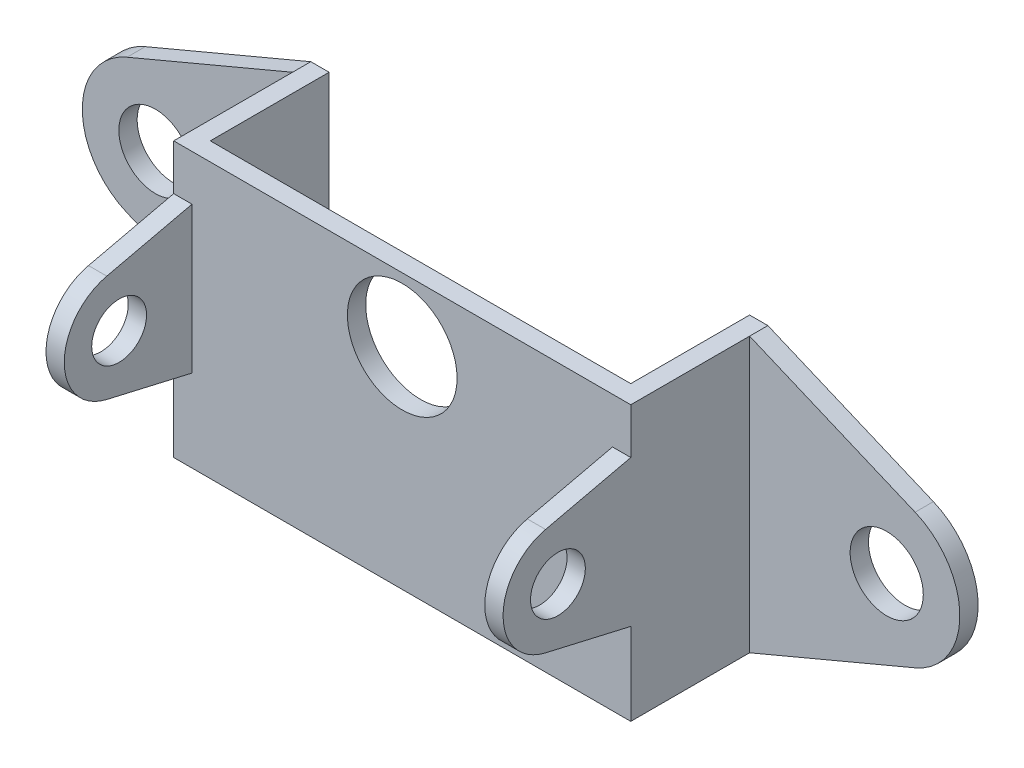
from build123d import *

# Parameters (mm, degrees)
SKETCH1_R             = 2
BOSS_EXTRUDE1_DEPTH   = 1
BOSS_EXTRUDE1_2_DEPTH = 1
SKETCH2_W             = 1
SKETCH2_H             = 15
BOSS_EXTRUDE2_DEPTH   = 6.5
SKETCH4_W             = 24.99999999
SKETCH4_H             = 15
SKETCH4_R             = 3
BOSS_EXTRUDE3_DEPTH   = 1
SKETCH6_R             = 1.5
BOSS_EXTRUDE4_DEPTH   = 1
CUT_EXTRUDE1_DEPTH    = 1
SKETCH8_R             = 1.5
BOSS_EXTRUDE5_DEPTH   = 1


with BuildPart() as part:
    # Sketch1 → Boss-Extrude1 (new body)
    with BuildSketch(Plane.XY):
        with BuildLine():
            Line((-99.978251459, 146.432775889), (-109.031169153, 142.619026916))
            Line((-109.031169153, 142.619026916), (-109.031169153, 157.619026916))
            Line((-109.031169153, 157.619026916), (-99.978251459, 153.805277943))
            ThreePointArc((-99.978251459, 153.805277943), (-97.531169153, 150.119026916), (-99.978251459, 146.432775889))
        make_face()
        with Locations((-101.531169153, 150.119026916)):
            Circle(SKETCH1_R, mode=Mode.SUBTRACT)
    extrude(amount=BOSS_EXTRUDE1_DEPTH)

    # Sketch2 → Boss-Extrude2 (add)
    with BuildSketch(Plane.XY):
        with Locations((-109.531169153, 150.119026916)):
            Rectangle(SKETCH2_W, SKETCH2_H)
        with Locations((-133.531169143, 150.119026916)):
            Rectangle(SKETCH2_W, SKETCH2_H)
    extrude(amount=BOSS_EXTRUDE2_DEPTH)


with BuildPart() as body_2:
    # Sketch1 → Boss-Extrude1 2 (new body)
    with BuildSketch(Plane.XY):
        with BuildLine():
            Line((-143.084086847, 153.805277943), (-134.031169153, 157.619026916))
            Line((-134.031169153, 157.619026916), (-134.031169153, 142.619026916))
            Line((-134.031169153, 142.619026916), (-143.084086847, 146.432775889))
            ThreePointArc((-143.084086847, 146.432775889), (-145.531169153, 150.119026916), (-143.084086847, 153.805277943))
        make_face()
        with Locations(Location((-141.531169153, 150.119026916, 0), (0, 0, 180))):
            Circle(SKETCH1_R, mode=Mode.SUBTRACT)
    extrude(amount=BOSS_EXTRUDE1_2_DEPTH)


with BuildPart() as boss_extrude2_piece_1:
    # of the separate pieces the step leaves, piece 1, a body of its own (boss_extrude2_pieces)
    add(part.part.solids().sort_by_distance((-99.978251459, 146.432775889, 0))[0])

    # Sketch4 → Boss-Extrude3 (add)
    with BuildSketch(Plane.XY.offset(6.5)):
        with Locations((-121.531169148, 150.119026916)):
            Rectangle(SKETCH4_W, SKETCH4_H)
        with Locations((-121.531169153, 154.119026916)):
            Circle(SKETCH4_R, mode=Mode.SUBTRACT)
    extrude(amount=BOSS_EXTRUDE3_DEPTH)



with BuildPart() as boss_extrude2_piece_2:
    # of the separate pieces the step leaves, piece 2, a body of its own (boss_extrude2_pieces)
    add(part.part.solids().sort_by_distance((-134.031169143, 157.619026916, 0))[0])


with BuildPart() as boss_extrude2_piece_1_1:
    add(boss_extrude2_piece_1.part)

    add(boss_extrude2_piece_2.part)  # Boss-Extrude4 merges Boss-Extrude2 piece 2
    # Sketch6 → Boss-Extrude4 (add)
    with BuildSketch(Plane.ZY.offset(134.031169143)):
        with BuildLine():
            Line((11.484935003, 147.119026916), (5.675712497, 147.119026916))
            ThreePointArc((5.675712497, 147.119026916), (1.675712497, 151.119026916), (5.675712497, 155.119026916))
            Line((5.675712497, 155.119026916), (11.484935003, 155.119026916))
            ThreePointArc((11.484935003, 155.119026916), (15.484935003, 151.119026916), (11.484935003, 147.119026916))
        make_face()
        with Locations((11.484935003, 151.119026916)):
            Circle(SKETCH6_R, mode=Mode.SUBTRACT)
    extrude(amount=-BOSS_EXTRUDE4_DEPTH)

    # Sketch7 → Cut-Extrude1 (cut)
    with BuildSketch(Plane.ZY.offset(134.031169143)):
        with BuildLine():
            Line((12.160438985, 154.041986781), (7.5, 155.119026916))
            Line((7.5, 155.119026916), (10.709914087, 160.89800408))
            Line((10.709914087, 160.89800408), (15.340416768, 156.67870434))
            Line((15.340416768, 156.67870434), (15.715862932, 151.386701277))
            Line((15.715862932, 151.386701277), (14.535889275, 146.058941435))
            Line((14.535889275, 146.058941435), (7.5, 147.119026916))
            Line((7.5, 147.119026916), (12.160438985, 148.196067051))
            ThreePointArc((12.160438985, 148.196067051), (14.484935003, 151.119026916), (12.160438985, 154.041986781))
        make_face()
    extrude(amount=-CUT_EXTRUDE1_DEPTH, mode=Mode.SUBTRACT)

    # Sketch8 → Boss-Extrude5 (add)
    with BuildSketch(Plane(origin=(-109.031169153, 0, 0), x_dir=(0, 0, -1), z_dir=(1, 0, 0))):
        with BuildLine():
            Line((-7.5, 147.119026916), (-7.5, 155.119026916))
            Line((-7.5, 155.119026916), (-12.160438985, 154.041986781))
            ThreePointArc((-12.160438985, 154.041986781), (-14.484935003, 151.119026916), (-12.160438985, 148.196067051))
            Line((-12.160438985, 148.196067051), (-7.5, 147.119026916))
        make_face()
        with Locations(Location((-11.484935003, 151.119026916, 0), (0, 0, 180))):
            Circle(SKETCH8_R, mode=Mode.SUBTRACT)
    extrude(amount=-BOSS_EXTRUDE5_DEPTH)


solid = Compound([body_2.part, boss_extrude2_piece_1_1.part])
